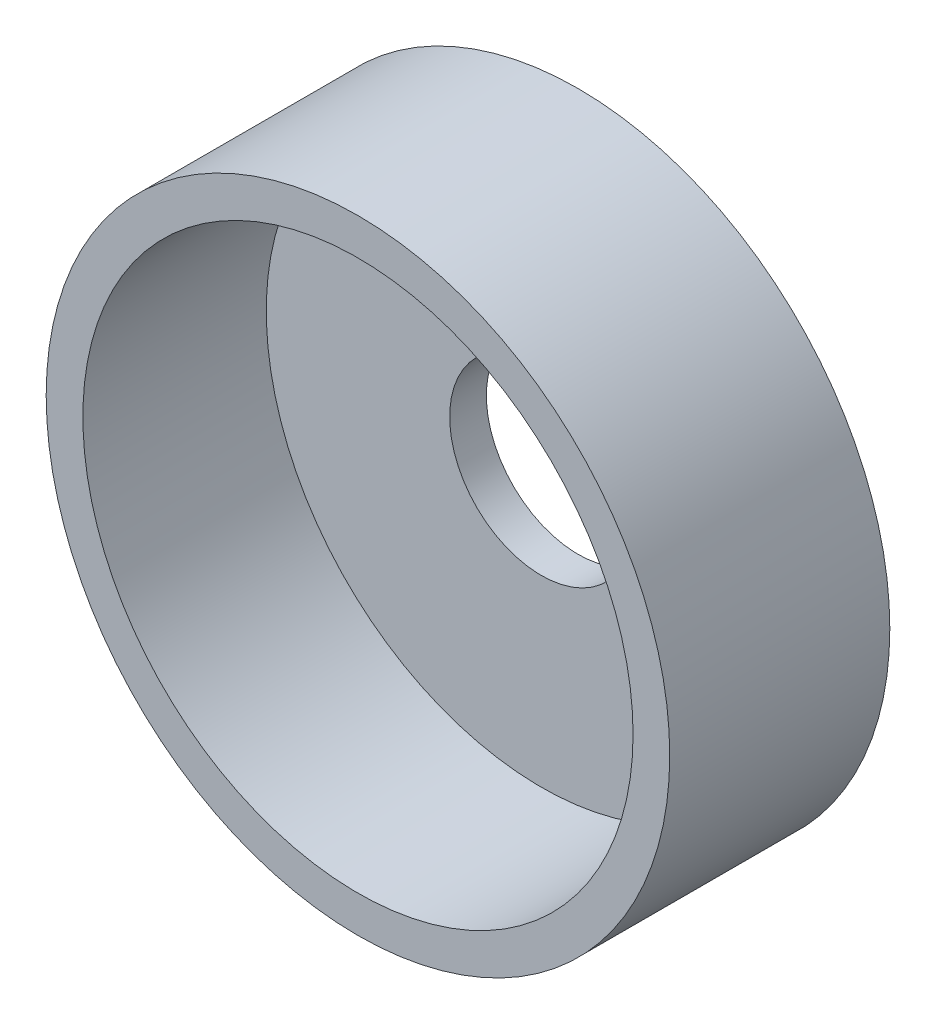
from build123d import *

# Parameters (mm, degrees)
SKETCH1_R           = 8.5
SKETCH1_R_2         = 2.5
BOSS_EXTRUDE1_DEPTH = 6
SKETCH2_R           = 7.5
CUT_EXTRUDE1_DEPTH  = 5


with BuildPart() as part:
    # Sketch1 → Boss-Extrude1 (new body)
    with BuildSketch(Plane.XY):
        Circle(SKETCH1_R)
        Circle(SKETCH1_R_2, mode=Mode.SUBTRACT)
    extrude(amount=BOSS_EXTRUDE1_DEPTH)

    # Sketch2 → Cut-Extrude1 (cut)
    with BuildSketch(Plane.XY.offset(6)):
        Circle(SKETCH2_R)
    extrude(amount=-CUT_EXTRUDE1_DEPTH, mode=Mode.SUBTRACT)


solid = part.part
